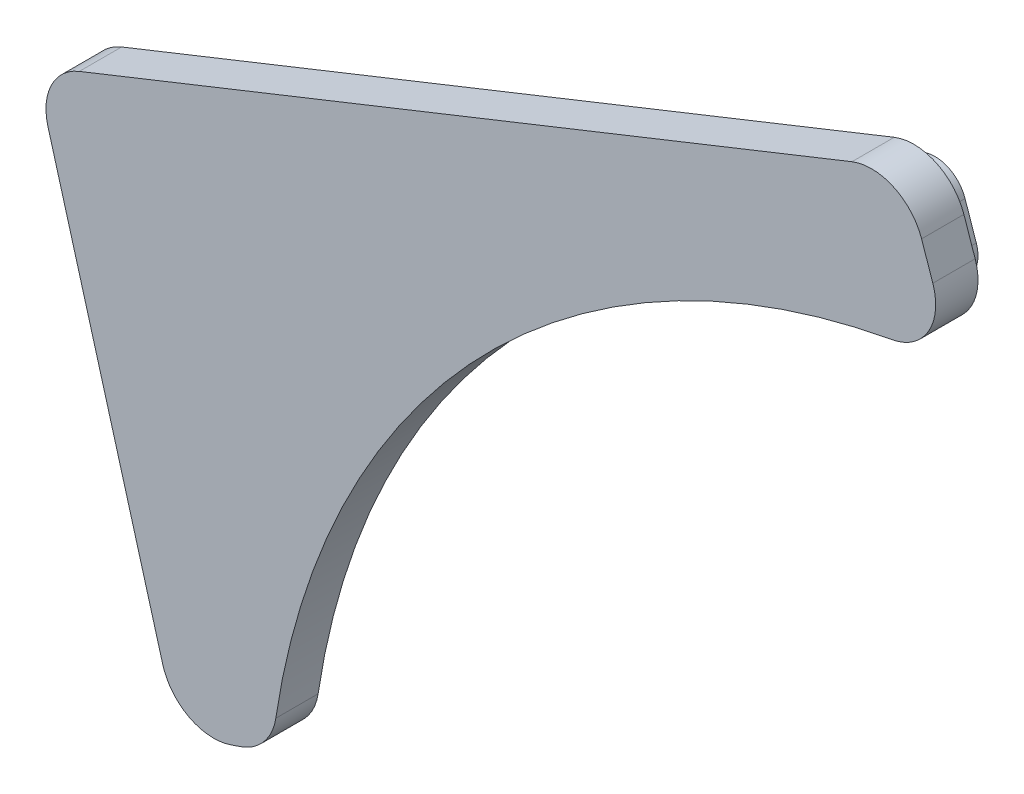
SolidWorks part; units mm, degrees
ref_plane "前视基准面" through (0, 0, 0) normal (0, 0, 1) x (1, 0, 0)
ref_plane "上视基准面" through (0, 0, 0) normal (0, 1, 0) x (1, 0, 0)
ref_plane "右视基准面" through (0, 0, 0) normal (1, 0, 0) x (0, 0, -1)
sketch "草图1" plane through (0, 0, 0) normal (0, 0, 1) x (1, 0, 0)
  line L0 (137.489, 148.5606) -> (148.3358, 109.9739) construction
  line L1 (152.1974, 107.9481) -> (153.1245, 108.2662) construction
  line L2 (212.2848, 181.2759) -> (139.2658, 152.159) construction
  line L3 (217.2976, 176.3615) -> (216.2336, 179.4628) construction
  line L4 (137.489, 148.5606) -> (148.3358, 109.9739)
  line L5 (152.1974, 107.9481) -> (153.1245, 108.2662)
  line L6 (212.2848, 181.2759) -> (139.2658, 152.159)
  line L7 (217.2976, 176.3615) -> (216.2336, 179.4628)
  arc A0 (139.2658, 152.159) -> (137.489, 148.5606) centre (140.377, 149.3724) ccw construction
  arc A1 (148.3358, 109.9739) -> (152.1974, 107.9481) centre (151.2239, 110.7858) ccw construction
  arc A2 (153.1245, 108.2662) -> (155.1176, 110.6572) centre (152.151, 111.1038) ccw construction
  arc A3 (214.9989, 172.4368) -> (155.1176, 110.6572) centre (228.293, 99.6407) ccw construction
  arc A4 (216.2336, 179.4628) -> (212.2848, 181.2759) centre (213.396, 178.4893) ccw construction
  arc A5 (214.9989, 172.4368) -> (217.2976, 176.3615) centre (214.4599, 175.388) ccw construction
  arc A6 (139.2658, 152.159) -> (137.489, 148.5606) centre (140.377, 149.3724) ccw
  arc A7 (148.3358, 109.9739) -> (152.1974, 107.9481) centre (151.2239, 110.7858) ccw
  arc A8 (153.1245, 108.2662) -> (155.1176, 110.6572) centre (152.151, 111.1038) ccw
  arc A9 (214.9989, 172.4368) -> (155.1176, 110.6572) centre (228.293, 99.6407) ccw
  arc A10 (216.2336, 179.4628) -> (212.2848, 181.2759) centre (213.396, 178.4893) ccw
  arc A11 (214.9989, 172.4368) -> (217.2976, 176.3615) centre (214.4599, 175.388) ccw
extrude "凸台-拉伸1" add sketch "草图1" against normal blind 2
sketch "草图2" plane through (0, 0, 0) normal (0, 0, 1) x (1, 0, 0)
  line L8 (154.5015, 74.3658) -> (160.1778, 76.31) construction
  line L9 (153.7735, 106.3744) -> (152.8464, 106.0563)
  line L10 (146.4104, 109.4327) -> (135.5636, 148.0193)
  line L11 (138.525, 154.0168) -> (211.544, 183.1336)
  line L12 (218.1254, 180.1118) -> (219.1894, 177.0105)
  arc A0 (268.537, 32.9371) -> (261.5, 35.7557) centre (263.806, 31.3192) ccw construction
  arc A1 (266.2514, 23.4123) -> (269.5979, 29.8347) centre (264.8669, 28.2169) ccw construction
  arc A2 (184.698, 4.5686) -> (190.7146, 1.6463) centre (189.3302, 6.4508) ccw construction
  arc A3 (172.6236, 48.3155) -> (169.6093, 41.7023) centre (174.2415, 43.5845) ccw construction
  arc A4 (178.6186, 47.5211) -> (173.5511, 48.6327) centre (175.1689, 43.9017) ccw construction
  arc A12 (157.0953, 110.3595) -> (215.3582, 170.4693) centre (228.293, 99.6407) cw
  arc A13 (157.0953, 110.3595) -> (153.7735, 106.3744) centre (152.151, 111.1038) cw
  arc A14 (152.8464, 106.0563) -> (146.4104, 109.4327) centre (151.2239, 110.7858) cw
  arc A15 (135.5636, 148.0193) -> (138.525, 154.0168) centre (140.377, 149.3724) cw
  arc A16 (211.544, 183.1336) -> (218.1254, 180.1118) centre (213.396, 178.4893) cw
  arc A17 (219.1894, 177.0105) -> (215.3582, 170.4693) centre (214.4599, 175.388) cw
extrude "凸台-拉伸2" add sketch "草图2" along normal blind 4
